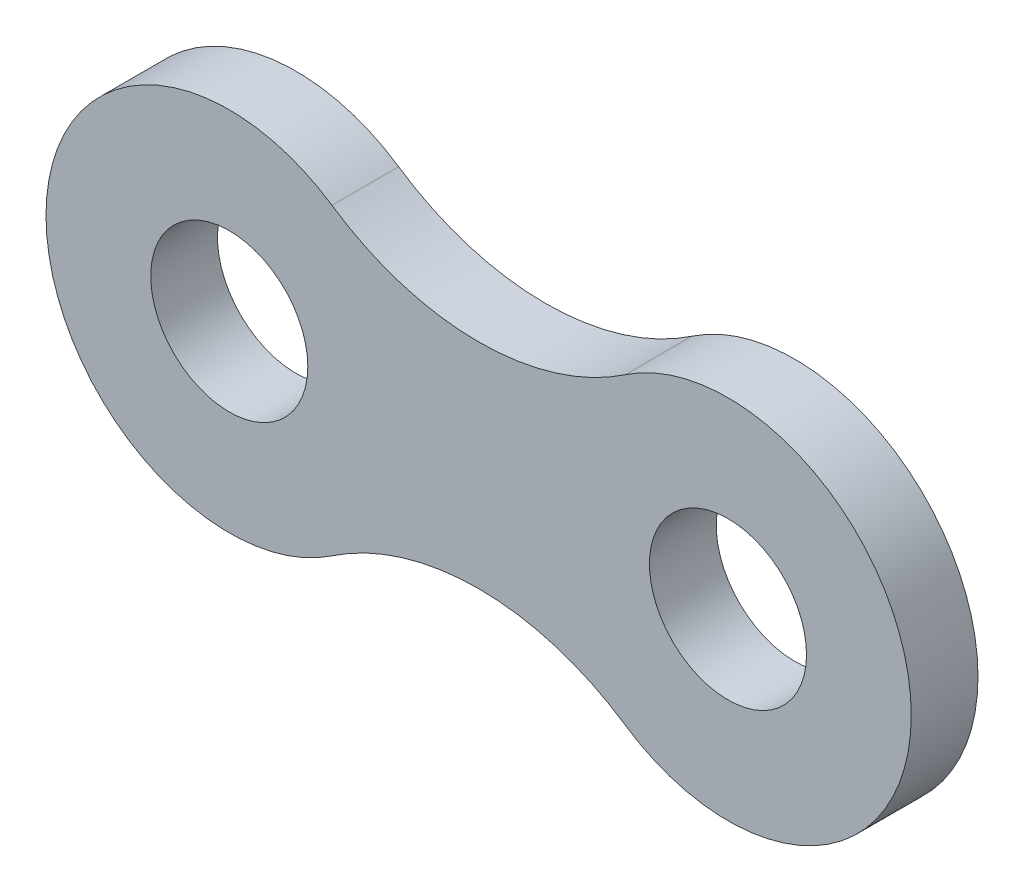
from build123d import *

# Parameters (mm, degrees)
SKETCH1_R           = 3
BOSS_EXTRUDE1_DEPTH = 2.55


with BuildPart() as part:
    # Sketch1 → Boss-Extrude1 (new body)
    with BuildSketch(Plane.XY):
        with BuildLine():
            ThreePointArc((3.922058824, 5.798056104), (-7, 0), (3.922058824, -5.798056104))
            ThreePointArc((3.922058824, -5.798056104), (9.525, -4.080993395), (15.127941176, -5.798056104))
            ThreePointArc((15.127941176, -5.798056104), (26.05, 0), (15.127941176, 5.798056104))
            ThreePointArc((15.127941176, 5.798056104), (9.525, 4.080993395), (3.922058824, 5.798056104))
        make_face()
        Circle(SKETCH1_R, mode=Mode.SUBTRACT)
        with Locations((19.05, 0)):
            Circle(SKETCH1_R, mode=Mode.SUBTRACT)
    extrude(amount=BOSS_EXTRUDE1_DEPTH)


solid = part.part
